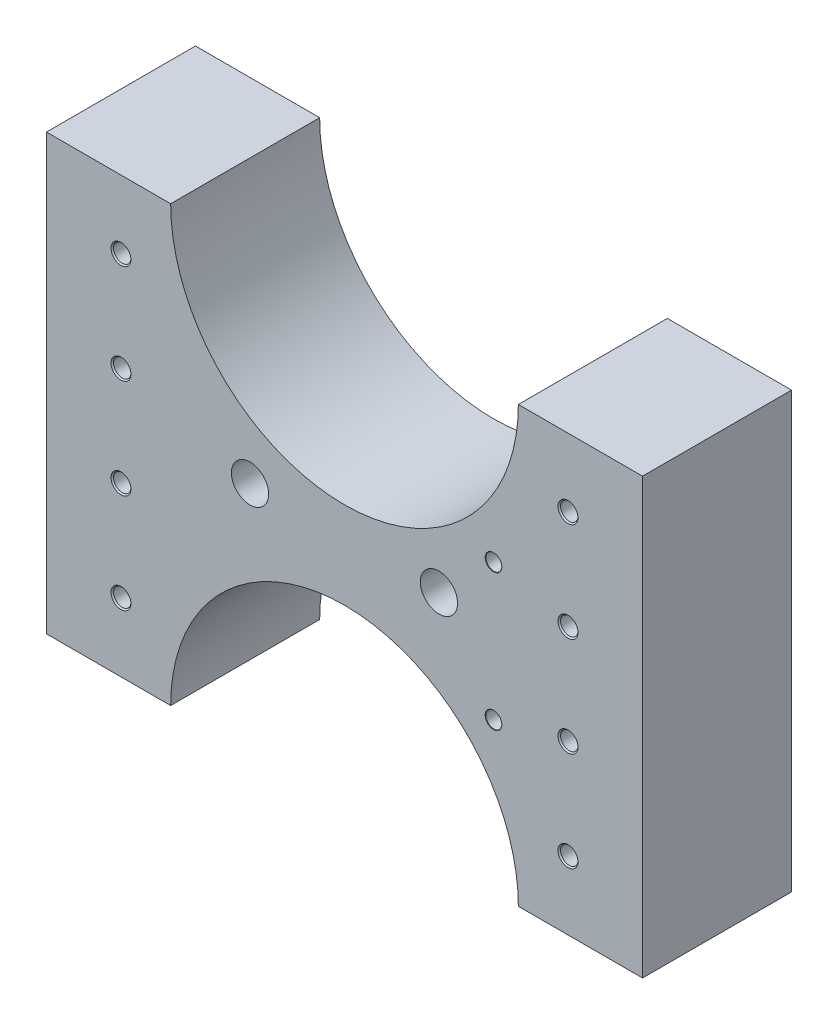
SolidWorks part; units mm, degrees
ref_plane "前视基准面" through (0, 0, 0) normal (0, 0, 1) x (1, 0, 0)
ref_plane "上视基准面" through (0, 0, 0) normal (0, 1, 0) x (1, 0, 0)
ref_plane "右视基准面" through (0, 0, 0) normal (1, 0, 0) x (0, 0, -1)
sketch "草图1" plane through (0, 0, 0) normal (0, 0, 1) x (1, 0, 0)
  line L0 (-140, -175) -> (-240, -175)
  line L1 (240, 175) -> (140, 175)
  line L2 (240, 175) -> (240, -175)
  line L3 (240, -175) -> (140, -175)
  line L4 (-240, 175) -> (-240, -175)
  line L5 (240, 175) -> (-240, -175) construction
  line L6 (240, -175) -> (-240, 175) construction
  line L7 (0, 0) -> (0, -175) construction
  line L8 (-140, -175) -> (140, -175) construction
  line L9 (0, 0) -> (240, 0) construction
  line L10 (-140, 175) -> (-240, 175)
  arc A0 (140, -175) -> (-140, -175) centre (0, -175) ccw
  arc A1 (140, 175) -> (-140, 175) centre (0, 175) cw
  point P0 (0, 0)
  dimension "D3" = 280
  dimension "D1" = 350
  dimension "D2" = 480
extrude "凸台-拉伸1" add sketch "草图1" along normal blind 120
hole_wizard "M16 螺纹孔1" positions "草图3" profile "草图4" tap size "M16" standard "GB"
sketch "草图3" plane through (0, 0, 120) normal (0, 0, 1) x (1, 0, 0)
  line L0 (-180, 192.1841) -> (-180, -214.3886) construction
  line L2 (0, 245.7813) -> (0, -251.141) construction
  line L4 (-140, 175) -> (-240, 175) construction
  point P0 (-180, 120)
  point P2 (-180, 40)
  point P4 (-180, -40)
  point P6 (-180, -120)
  point P25 (180, -120)
  point P26 (180, -40)
  point P27 (180, 40)
  point P28 (180, 120)
  dimension "D1" = 180
  dimension "D2" = 55
  dimension "D3" = 80
  dimension "D4" = 80
  dimension "D5" = 80
sketch "草图4" plane through (-180, 120, 120) normal (1, 0, 0) x (0, -1, 0)
  line L0 (0, 0) -> (0, 36)
  line L1 (0, 36) -> (7, 31.794)
  line L2 (7, 31.794) -> (7, 1.025)
  line L3 (7, 1.025) -> (8.025, 0)
  line L5 (8.025, 0) -> (0, 0)
  line L6 (-7, 1.025) -> (-8.025, 0) construction
  line L10 (0, 36) -> (-7, 31.794) construction
  line L11 (0, -6.35) -> (0, 107.95) construction
  dimension "螺纹孔钻头直径" = 14
  dimension "螺纹孔钻头深度" = 36
  dimension "近端锥形沉头孔直径" = 16.05
  dimension "近端锥形沉头孔角度" = 90
  dimension "导头角度" = 118
cosmetic thread "孔螺蚊线1" parameters "D1"=30, "D2"=16
cosmetic thread "孔螺蚊线2" parameters "D1"=30, "D2"=16
cosmetic thread "孔螺蚊线3" parameters "D1"=30, "D2"=16
cosmetic thread "孔螺蚊线4" parameters "D1"=30, "D2"=16
cosmetic thread "孔螺蚊线5" parameters "D1"=30, "D2"=16
cosmetic thread "孔螺蚊线6" parameters "D1"=30, "D2"=16
cosmetic thread "孔螺蚊线7" parameters "D1"=30, "D2"=16
cosmetic thread "孔螺蚊线8" parameters "D1"=30, "D2"=16
sketch "草图5" plane through (0, 0, 120) normal (0, 0, 1) x (1, 0, 0)
  line L0 (-140, 175) -> (140, 175) construction
  line L1 (0, 0) -> (0, 35) construction
  line L2 (-76.0713, 11.8646) -> (0, 175) construction
  circle A0 centre (0, 175) radius 180 construction
  circle A1 centre (-76.0713, 11.8646) radius 15
  arc A2 (-140, 175) -> (140, 175) centre (0, 175) ccw construction
  circle A3 centre (76.0713, 11.8646) radius 15
  dimension "D1" = 360
  dimension "D2" = 30
  dimension "D3" = 25
extrude "切除-拉伸1" cut sketch "草图5" against normal through all both and the other way through all
sketch "草图6" plane through (0, 0, 120) normal (0, 0, 1) x (1, 0, 0)
  line L0 (0, 179.9333) -> (0, -189.5042) construction
  line L1 (240, 175) -> (140, 175) construction
  line L2 (140, -175) -> (240, -175) construction
  circle A0 centre (120, 55) radius 4
  circle A1 centre (120, -55) radius 4
  dimension "D5" = 8
  dimension "D6" = 8
  dimension "D1" = 120
  dimension "D2" = 120
  dimension "D3" = 120
  dimension "D4" = 120
extrude "切除-拉伸2" cut sketch "草图6" against normal through all both and the other way through all
hole_wizard "1/4 Rc 螺纹孔1" positions "草图7" profile "草图8" size "1/4" standard "GB"
sketch "草图7" plane through (0, 0, 120) normal (0, 0, 1) x (1, 0, 0)
  point P0 (120, 55)
  point P3 (120, -55)
sketch "草图8" plane through (120, 55, 120) normal (1, 0, 0) x (0, -1, 0)
  line L0 (0, 0) -> (0, 20)
  line L1 (5.35, 16.7854) -> (0, 20)
  line L2 (-5.35, 16.7854) -> (0, 20) construction
  line L3 (5.35, 16.7854) -> (5.35, 20)
  line L4 (5.35, 20) -> (5.8186, 20)
  line L5 (5.8186, 20) -> (6.4349, 0.2551)
  line L6 (6.4349, 0.2551) -> (6.69, 0)
  line L7 (6.69, 0) -> (0, 0)
  line L8 (0, -6.35) -> (0, 107.95) construction
  line L9 (-6.4349, 0.2551) -> (-6.69, 0) construction
  line L11 (-5.35, 20) -> (-5.8186, 20) construction
  line L12 (-5.8186, 20) -> (-6.4349, 0.2551) construction
  dimension "螺纹孔钻头直径" = 10.7
  dimension "螺纹孔钻头深度" = 20
  dimension "螺纹直径" = 12.8699
  dimension "螺纹角度" = 3.576
  dimension "螺纹深度" = 20
  dimension "锥形沉头孔直径" = 13.38
  dimension "锥形沉头孔角度" = 90
  dimension "导头角度" = 118
cosmetic thread "孔螺蚊线9" parameters "D1"=20, "D2"=13.7329
cosmetic thread "孔螺蚊线10" parameters "D1"=20, "D2"=13.7329
hole_wizard "1/4 Rc 螺纹孔2" positions "草图9" profile "草图10" size "1/4" standard "GB"
sketch "草图9" plane through (0, 0, 0) normal (0, 0, -1) x (-1, 0, 0)
  point P0 (-120, 55)
  point P3 (-120, -55)
sketch "草图10" plane through (120, 55, 0) normal (1, 0, 0) x (0, 1, 0)
  line L0 (0, 0) -> (0, 20)
  line L1 (5.35, 16.7854) -> (0, 20)
  line L2 (-5.35, 16.7854) -> (0, 20) construction
  line L3 (5.35, 16.7854) -> (5.35, 20)
  line L4 (5.35, 20) -> (5.8186, 20)
  line L5 (5.8186, 20) -> (6.4349, 0.2551)
  line L6 (6.4349, 0.2551) -> (6.69, 0)
  line L7 (6.69, 0) -> (0, 0)
  line L8 (0, -6.35) -> (0, 107.95) construction
  line L9 (-6.4349, 0.2551) -> (-6.69, 0) construction
  line L11 (-5.35, 20) -> (-5.8186, 20) construction
  line L12 (-5.8186, 20) -> (-6.4349, 0.2551) construction
  dimension "螺纹孔钻头直径" = 10.7
  dimension "螺纹孔钻头深度" = 20
  dimension "螺纹直径" = 12.8699
  dimension "螺纹角度" = 3.576
  dimension "螺纹深度" = 20
  dimension "锥形沉头孔直径" = 13.38
  dimension "锥形沉头孔角度" = 90
  dimension "导头角度" = 118
cosmetic thread "孔螺蚊线11" parameters "D1"=20, "D2"=13.7329
cosmetic thread "孔螺蚊线12" parameters "D1"=20, "D2"=13.7329
ref_plane "基准面1" through (-17.5, -17.5, 0) normal (-0.7071, -0.7071, 0) x (0, 0, -1)
sketch "草图12" plane through (-17.5, -17.5, 0) normal (-0.7071, -0.7071, 0) x (0, 0, -1)
  line L0 (-60, 222.7386) -> (-60, 24.7487) construction
  line L1 (-120, 222.7386) -> (0, 222.7386) construction
  line L2 (-120, 24.7487) -> (0, 24.7487) construction
  line L3 (0, 222.7386) -> (0, 24.7487) construction
  line L4 (0, 123.7437) -> (-120, 123.7437) construction
  line L5 (-120, 222.7386) -> (-120, -16.2563) construction
  circle A0 centre (-60, 123.7437) radius 4
  dimension "D1" = 8
extrude "切除-拉伸3" cut sketch "草图12" against normal up to next
sketch "草图14" plane through (-17.5, -17.5, 0) normal (-0.7071, -0.7071, 0) x (0, 0, -1)
  circle A0 centre (-60, 123.7437) radius 12.5
  dimension "D1" = 25
extrude "切除-拉伸4" cut sketch "草图14" against normal blind 44.01
mirror "镜向1" about plane through (0, 0, 0) normal (0, 1, 0) of "切除-拉伸4", "切除-拉伸3"
